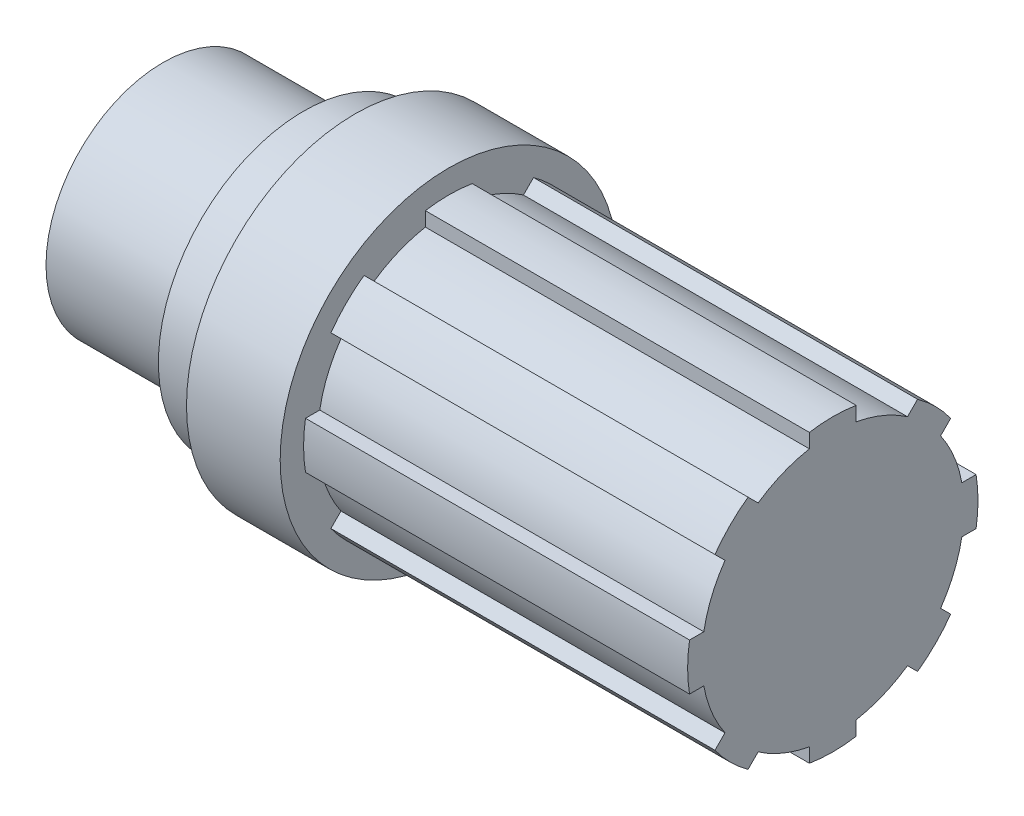
SolidWorks part; units mm, degrees
material "6061"
ref_plane "Front Plane" through (0, 0, 0) normal (0, 0, 1) x (1, 0, 0)
ref_plane "Top Plane" through (0, 0, 0) normal (0, 1, 0) x (1, 0, 0)
ref_plane "Right Plane" through (0, 0, 0) normal (1, 0, 0) x (0, 0, -1)
sketch "Sketch1" plane through (0, 0, 0) normal (0, 1, 0) x (1, 0, 0)
  line L0 (0, 0) -> (0, 31)
  line L1 (0, 31) -> (11, 31)
  line L2 (11, 31) -> (11, 36)
  line L3 (11, 36) -> (31, 36)
  line L4 (31, 36) -> (31, 28)
  line L5 (31, 28) -> (113, 28)
  line L6 (113, 28) -> (113, 0)
  line L7 (113, 0) -> (0, 0) construction
  line L8 (0, 0) -> (113, 0)
  dimension "D1" = 62
  dimension "D2" = 31
  dimension "D3" = 11
  dimension "D4" = 5
  dimension "D5" = 113
  dimension "D6" = 28
revolve "Revolve1" add sketch "Sketch1" angle 360 about L7
sketch "Sketch2" plane through (113, 0, 0) normal (1, 0, 0) x (0, 0, -1)
  line L0 (0, 0) -> (0, 28) construction
  line L3 (-5, 30.5941) -> (-5, 27.55)
  line L5 (5, 30.5941) -> (5, 27.55)
  arc A0 (-5, 27.55) -> (5, 27.55) centre (0, 0) cw
  arc A4 (5, 30.5941) -> (-5, 30.5941) centre (0, 0) ccw
  dimension "D3" = 28
  dimension "D1" = 31
  dimension "D2" = 10
extrude "Boss-Extrude1" add sketch "Sketch2" against normal up to surface (82 mm away) up to face at (31, 0, -36)
pattern_circular "CirPattern1" count 8 over 360 about axis through (0, 0, 0) along (1, 0, 0) of "Boss-Extrude1"
sketch "Sketch3" plane through (0, 0, 0) normal (-1, 0, 0) x (0, 0, 1)
  circle A0 centre (0, 0) radius 25
  dimension "D1" = 50
extrude "Boss-Extrude2" add sketch "Sketch3" along normal blind 30
